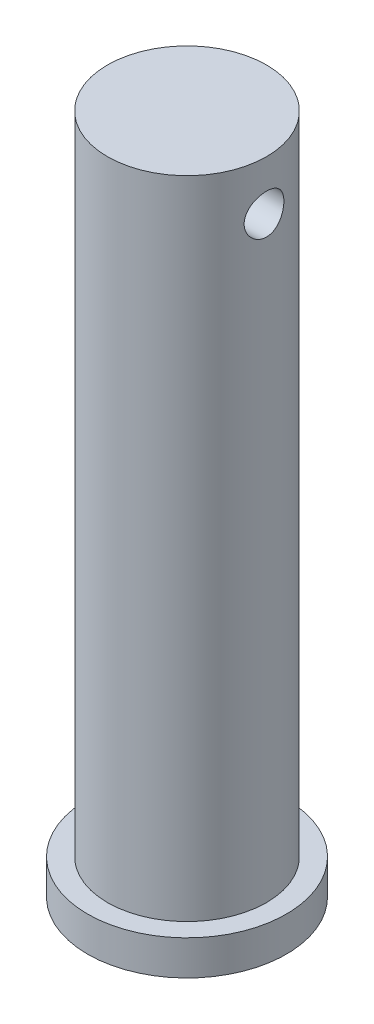
SolidWorks part; units mm, degrees
ref_plane "前视基准面" through (0, 0, 0) normal (0, 0, 1) x (1, 0, 0)
ref_plane "上视基准面" through (0, 0, 0) normal (0, 1, 0) x (1, 0, 0)
ref_plane "右视基准面" through (0, 0, 0) normal (1, 0, 0) x (0, 0, -1)
sketch "草图1" plane through (0, 0, 0) normal (0, 0, 1) x (1, 0, 0)
  line L0 (0, 34.25) -> (0, -34.25)
  line L1 (0, -34.25) -> (10, -34.25)
  line L2 (10, -34.25) -> (10, -30.75)
  line L3 (10, -30.75) -> (8, -30.75)
  line L4 (8, -30.75) -> (8, 34.25)
  line L5 (8, 34.25) -> (0, 34.25)
  point P4 (0, 0)
  dimension "D1" = 68.5
  dimension "D2" = 10
  dimension "D3" = 8
  dimension "D4" = 3.5
revolve "旋转1" add sketch "草图1" angle 360 about L0
sketch "草图2" plane through (0, 0, 0) normal (1, 0, 0) x (0, 0, -1)
  line L0 (8, 34.25) -> (-8, 34.25) construction
  circle A0 centre (0, 29.25) radius 2
  point P4 (0, 0)
  dimension "D1" = 4
  dimension "D2" = 5
extrude "切除-拉伸1" cut sketch "草图2" against normal mid plane 20
